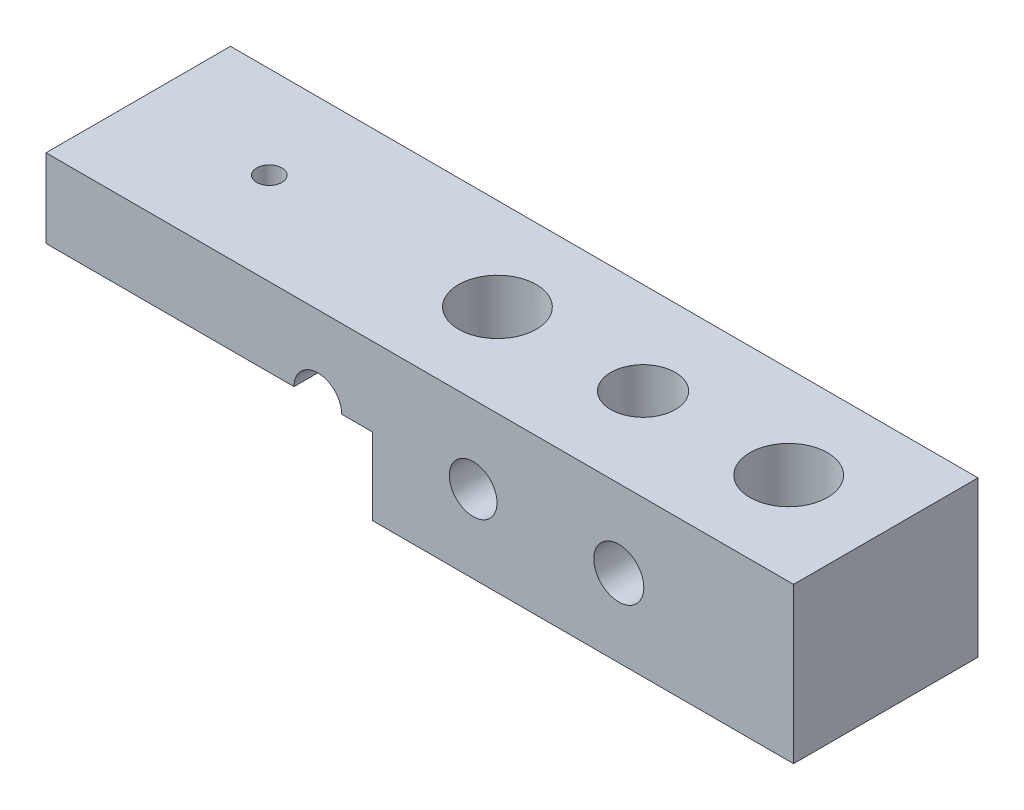
SolidWorks part; units mm, degrees
ref_plane "Front Plane" through (0, 0, 0) normal (0, 0, 1) x (1, 0, 0)
ref_plane "Top Plane" through (0, 0, 0) normal (0, 1, 0) x (1, 0, 0)
ref_plane "Right Plane" through (0, 0, 0) normal (1, 0, 0) x (0, 0, -1)
sketch "Sketch1" plane through (0, 0, 0) normal (0, 0, 1) x (1, 0, 0)
  line L0 (0, 0) -> (25.5415, 0)
  line L1 (33.6375, 0) -> (33.6375, -7.9074)
  line L2 (33.6375, -7.9074) -> (77, -7.9074)
  line L3 (77, -7.9074) -> (77, 8.0926)
  line L4 (77, 8.0926) -> (0, 8.0926)
  line L5 (0, 8.0926) -> (0, 0)
  line L6 (30.4585, 0) -> (33.6375, 0)
  line L7 (77, 0.0926) -> (35.5912, 0.0926) construction
  arc A0 (30.4585, 0) -> (25.5415, 0) centre (28, 0) ccw
  circle A1 centre (59, 0.0926) radius 2.5765
  circle A2 centre (44, 0.0926) radius 2.4585
  dimension "D5" = 5.6375
  dimension "D6" = 18
  dimension "D7" = 15
  dimension "D1" = 77
  dimension "D2" = 16
  dimension "D3" = 8.0926
  dimension "D4" = 43.3625
extrude "Boss-Extrude1" add sketch "Sketch1" along normal blind 19
ref_plane "Plane1" through (0, 8.0926, 0) normal (0, 1, 0) x (1, 0, 0)
sketch "Sketch2" plane through (0, 8.0926, 0) normal (0, 1, 0) x (1, 0, 0)
  line L0 (0, -9.5) -> (77, -9.5) construction
  line L1 (0, -19) -> (0, 0) construction
  line L2 (77, -19) -> (77, 0) construction
  circle A0 centre (67, -9.5) radius 4
  circle A1 centre (52, -9.5) radius 3.3235
  circle A2 centre (37, -9.5) radius 4
  circle A3 centre (13.5, -9.5) radius 1.2995
  dimension "D1" = 10
  dimension "D2" = 15
  dimension "D3" = 15
  dimension "D4" = 23.5
extrude "Cut-Extrude1" cut sketch "Sketch2" against normal through all
ref_plane "Plane2" through (0, 0, 0) normal (0, -1, 0) x (-1, 0, 0)
sketch "Sketch3" plane through (0, 0, 0) normal (0, -1, 0) x (-1, 0, 0)
  circle A0 centre (-13.5, -9.5) radius 5
extrude "Cut-Extrude2" cut sketch "Sketch3" against normal blind 5
